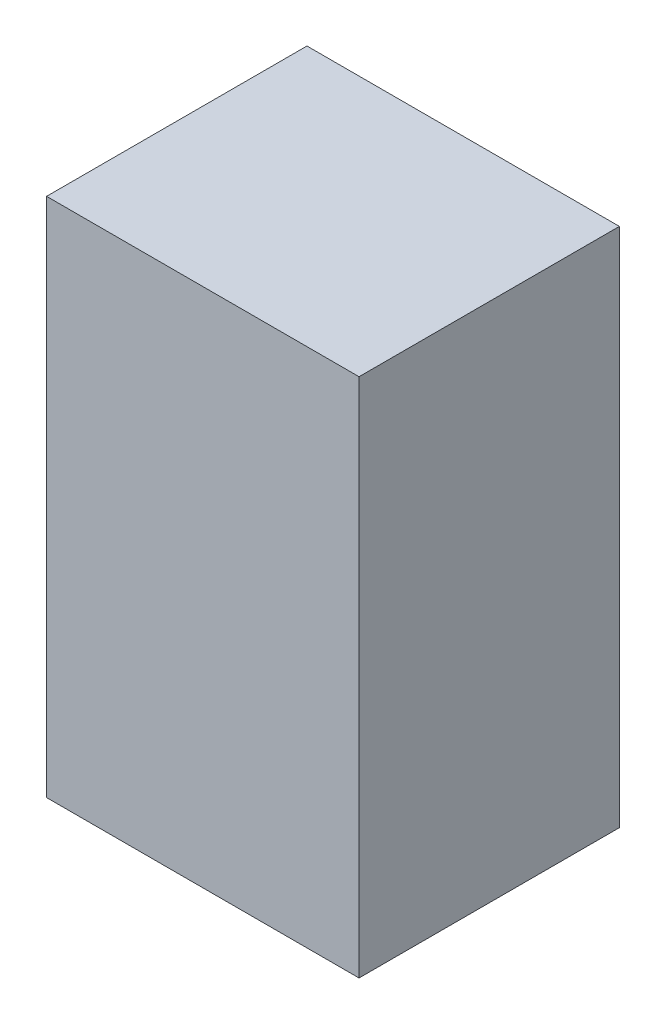
from build123d import *

# Parameters (mm, degrees)
SKETCH1_W           = 30
SKETCH1_H           = 50
BOSS_EXTRUDE1_DEPTH = 25


with BuildPart() as part:
    # Sketch1 → Boss-Extrude1 (new body)
    with BuildSketch(Plane.XY):
        with Locations((15, 25)):
            Rectangle(SKETCH1_W, SKETCH1_H)
    extrude(amount=BOSS_EXTRUDE1_DEPTH)


solid = part.part
